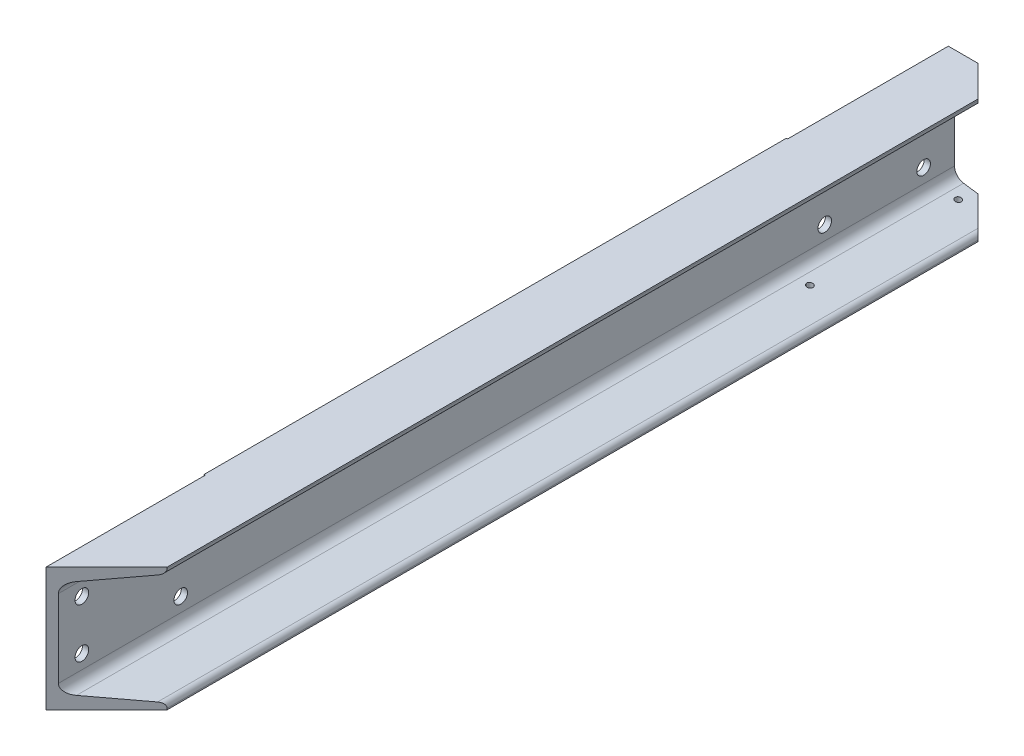
from build123d import *

# Parameters (mm, degrees)
BOSS_EXTRUDE1_DEPTH   = 750
CUT_EXTRUDE1_DEPTH    = 730
SKETCH3_W             = 246.792493201
SKETCH3_H             = 411.477698095
CUT_EXTRUDE2_DEPTH    = 1
SKETCH4_R             = 5.5
CUT_EXTRUDE3_DEPTH    = 10
M6_TAPPED_HOLE1_D     = 5
M6_TAPPED_HOLE1_DEPTH = 15
M6_TAPPED_HOLE1_TIP   = 1.502151548
M6_TAPPED_HOLE2_D     = 5
M6_TAPPED_HOLE2_DEPTH = 15
M6_TAPPED_HOLE2_TIP   = 1.502151548


with BuildPart() as part:
    # Sketch1 → Boss-Extrude1 (new body)
    with BuildSketch(Plane.XY):
        with BuildLine():
            Line((0, 0), (0, -100))
            Line((0, -100), (50, -100))
            Line((50, -100), (50, -98.925311188))
            ThreePointArc((50, -98.925311188), (48.896193111, -95.973045557), (46.126278954, -94.469104878))
            Line((46.126278954, -94.469104878), (13.317028642, -89.858065454))
            ThreePointArc((13.317028642, -89.858065454), (8.084968568, -87.017288616), (6, -81.440786869))
            Line((6, -81.440786869), (6, -18.559213131))
            ThreePointArc((6, -18.559213131), (8.084968568, -12.982711384), (13.317028642, -10.141934546))
            Line((13.317028642, -10.141934546), (46.126278954, -5.530895122))
            ThreePointArc((46.126278954, -5.530895122), (48.896193111, -4.026954443), (50, -1.074688812))
            Line((50, -1.074688812), (50, 0))
            Line((50, 0), (0, 0))
        make_face()
    extrude(amount=BOSS_EXTRUDE1_DEPTH)

    # Sketch2 → Cut-Extrude1 (cut)
    with BuildSketch(Plane(origin=(0, 0, 0), x_dir=(1, 0, 0), z_dir=(0, 1, 0))):
        Polygon((258.992644717, -472.007355283), (0, -731), (-59.777153602, -772.262203455), (30.841373369, -818.159898935), (45.044802943, -785.872759949), (459.456990019, -587.675626999), align=None)
        Polygon((25, 0), (50, -25), (50, 48.41721094), align=None)
    extrude(amount=-CUT_EXTRUDE1_DEPTH, mode=Mode.SUBTRACT)

    # Sketch3 → Cut-Extrude2 (cut)
    with BuildSketch(Plane.ZY):
        Polygon((130, 38.70177923), (130, -162.725177772), (-125.633599865, -119.606257313), (-100.418312462, 29.884375145), align=None)
        with Locations((724.396246601, 67.037069817)):
            Rectangle(SKETCH3_W, SKETCH3_H)
    extrude(amount=-CUT_EXTRUDE2_DEPTH, mode=Mode.SUBTRACT)

    # Sketch4 → Cut-Extrude3 (cut)
    with BuildSketch(Plane.ZY.offset(-1)):
        with Locations(Location((25, -30, 0), (0, 0, 270))):
            Circle(SKETCH4_R)
        with Locations(Location((105, -30, 0), (0, 0, 270))):
            Circle(SKETCH4_R)
        with Locations(Location((25, -70, 0), (0, 0, 270))):
            Circle(SKETCH4_R)
        with Locations(Location((105, -70, 0), (0, 0, 270))):
            Circle(SKETCH4_R)
        with Locations(Location((626, -30, 0), (0, 0, 270))):
            Circle(SKETCH4_R)
        with Locations(Location((706, -70, 0), (0, 0, 270))):
            Circle(SKETCH4_R)
        with Locations(Location((626, -70, 0), (0, 0, 270))):
            Circle(SKETCH4_R)
        with Locations(Location((706, -30, 0), (0, 0, 270))):
            Circle(SKETCH4_R)
    extrude(amount=-CUT_EXTRUDE3_DEPTH, mode=Mode.SUBTRACT)

    # M6 Tapped Hole1
    with Locations(Plane(origin=(0, -100, 0), x_dir=(-1, 0, 0), z_dir=(0, -1, 0))):
        with Locations((-21.5, -12.5)):
            Hole(M6_TAPPED_HOLE1_D / 2, depth=M6_TAPPED_HOLE1_DEPTH)
            with Locations((0, 0, -(M6_TAPPED_HOLE1_DEPTH + M6_TAPPED_HOLE1_TIP / 2))):  # 118° drill point
                Cone(0, M6_TAPPED_HOLE1_D / 2, M6_TAPPED_HOLE1_TIP, mode=Mode.SUBTRACT)

    # M6 Tapped Hole2
    with Locations(Plane(origin=(0, -100, 0), x_dir=(-1, 0, 0), z_dir=(0, -1, 0))):
        with Locations((-21.5, -132.5)):
            Hole(M6_TAPPED_HOLE2_D / 2, depth=M6_TAPPED_HOLE2_DEPTH)
            with Locations((0, 0, -(M6_TAPPED_HOLE2_DEPTH + M6_TAPPED_HOLE2_TIP / 2))):  # 118° drill point
                Cone(0, M6_TAPPED_HOLE2_D / 2, M6_TAPPED_HOLE2_TIP, mode=Mode.SUBTRACT)


solid = part.part
